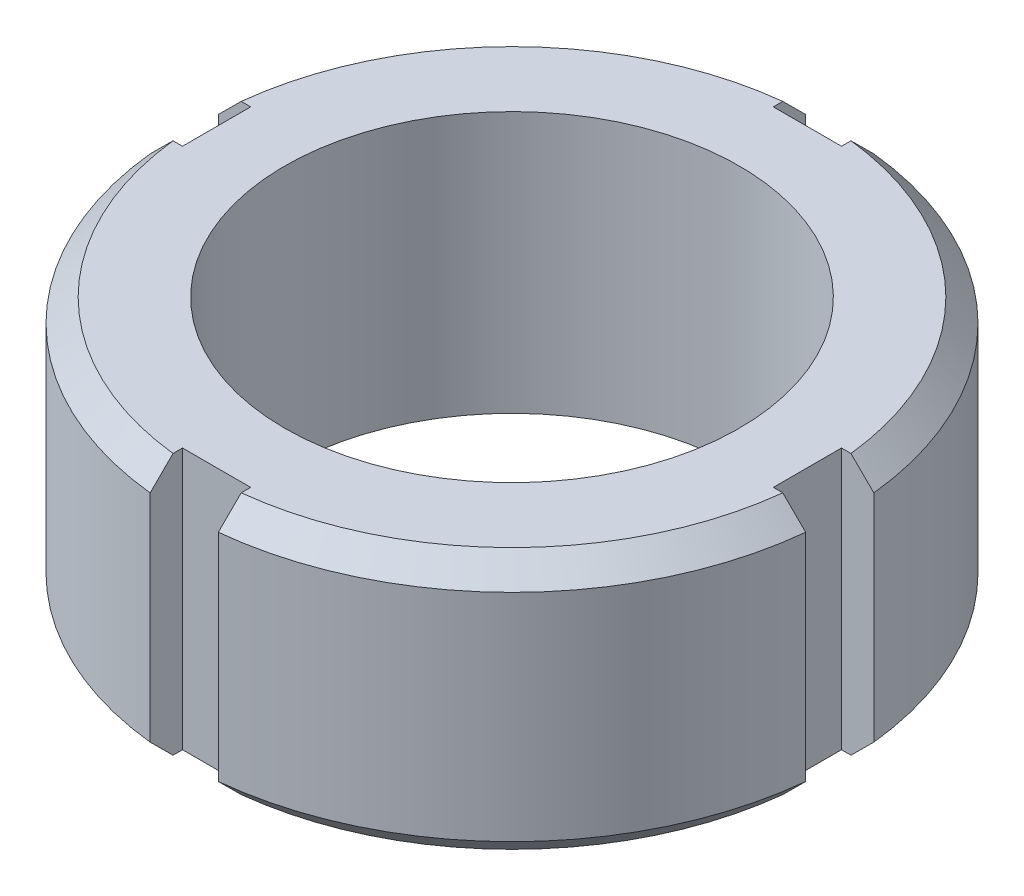
SolidWorks part; units mm, degrees
material "普通碳钢"
ref_plane "Front Plane" through (0, 0, 0) normal (0, 0, 1) x (1, 0, 0)
ref_plane "Top Plane" through (0, 0, 0) normal (0, 1, 0) x (1, 0, 0)
ref_plane "Right Plane" through (0, 0, 0) normal (1, 0, 0) x (0, 0, -1)
sketch "Sketch1" plane through (0, 0, 0) normal (0, 1, 0) x (1, 0, 0)
  circle A0 centre (0, 0) radius 20
  circle A1 centre (0, 0) radius 29
  dimension "D1" = 40
  dimension "D2" = 58
extrude "Boss-Extrude1" add sketch "Sketch1" along normal blind 23
cosmetic thread "Cosmetic Thread1" parameters "D2"=45
chamfer "Chamfer1" distance 2 angle 45 2 edges at (0, 0, 29) (0, 23, 29)
sketch "Sketch2" plane through (0, 23, 0) normal (0, 1, 0) x (1, 0, 0)
  line L1 (-3, 38.4368) -> (3, 38.4368)
  line L2 (-3, 38.4368) -> (-3, 26)
  line L3 (-3, 26) -> (3, 26)
  line L4 (3, 38.4368) -> (3, 26)
  dimension "D1" = 6
  dimension "D2" = 3
  dimension "D3" = 26
extrude "Cut-Extrude1" cut sketch "Sketch2" against normal through all
pattern_circular "CirPattern1" count 4 over 360 about axis through (0, 0, 0) along (0, 1, 0) of "Cut-Extrude1"
